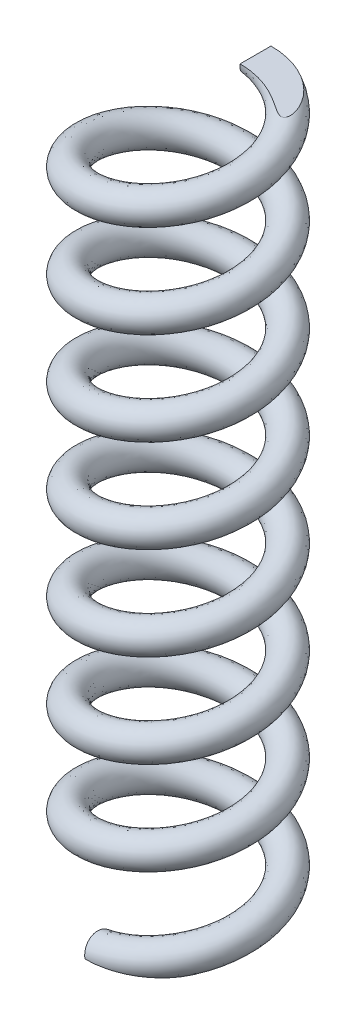
from build123d import *

# Parameters (mm, degrees)
SWEEP2_PITCH        = 6
SWEEP2_HEIGHT       = 45
SWEEP2_RADIUS       = 5
SKETCH5_R           = 1
SKETCH6_OUTSIDE_W   = 23.988
SKETCH6_OUTSIDE_H   = 58.952
SKETCH6_OUTSIDE_W_2 = 18
SKETCH6_OUTSIDE_H_2 = 45
END_GROUND_DEPTH    = 9


with BuildPart() as part:
    # Sweep2: sweep along a helix
    with BuildLine() as sweep2_path:
        Helix(SWEEP2_PITCH, SWEEP2_HEIGHT, SWEEP2_RADIUS, center=(0, 0, 0), direction=(0, 1, 0))
    # Sketch5 → Sweep2 (sweep)
    with BuildSketch(Plane(origin=(0, 0, 5), x_dir=(0, 0, -1), z_dir=(0.9822464167783632, 0.1875952470774938, 0))):
        Circle(SKETCH5_R)
    sweep(path=sweep2_path.line, is_frenet=True)

    # Sketch6 outside → End Ground (cut, symmetric)
    with BuildSketch(Plane.XY):
        with Locations((0, 22.5)):
            Rectangle(SKETCH6_OUTSIDE_W, SKETCH6_OUTSIDE_H)
        with Locations((0, 22.5)):
            Rectangle(SKETCH6_OUTSIDE_W_2, SKETCH6_OUTSIDE_H_2, mode=Mode.SUBTRACT)
    extrude(amount=END_GROUND_DEPTH, both=True, mode=Mode.SUBTRACT)


solid = part.part
